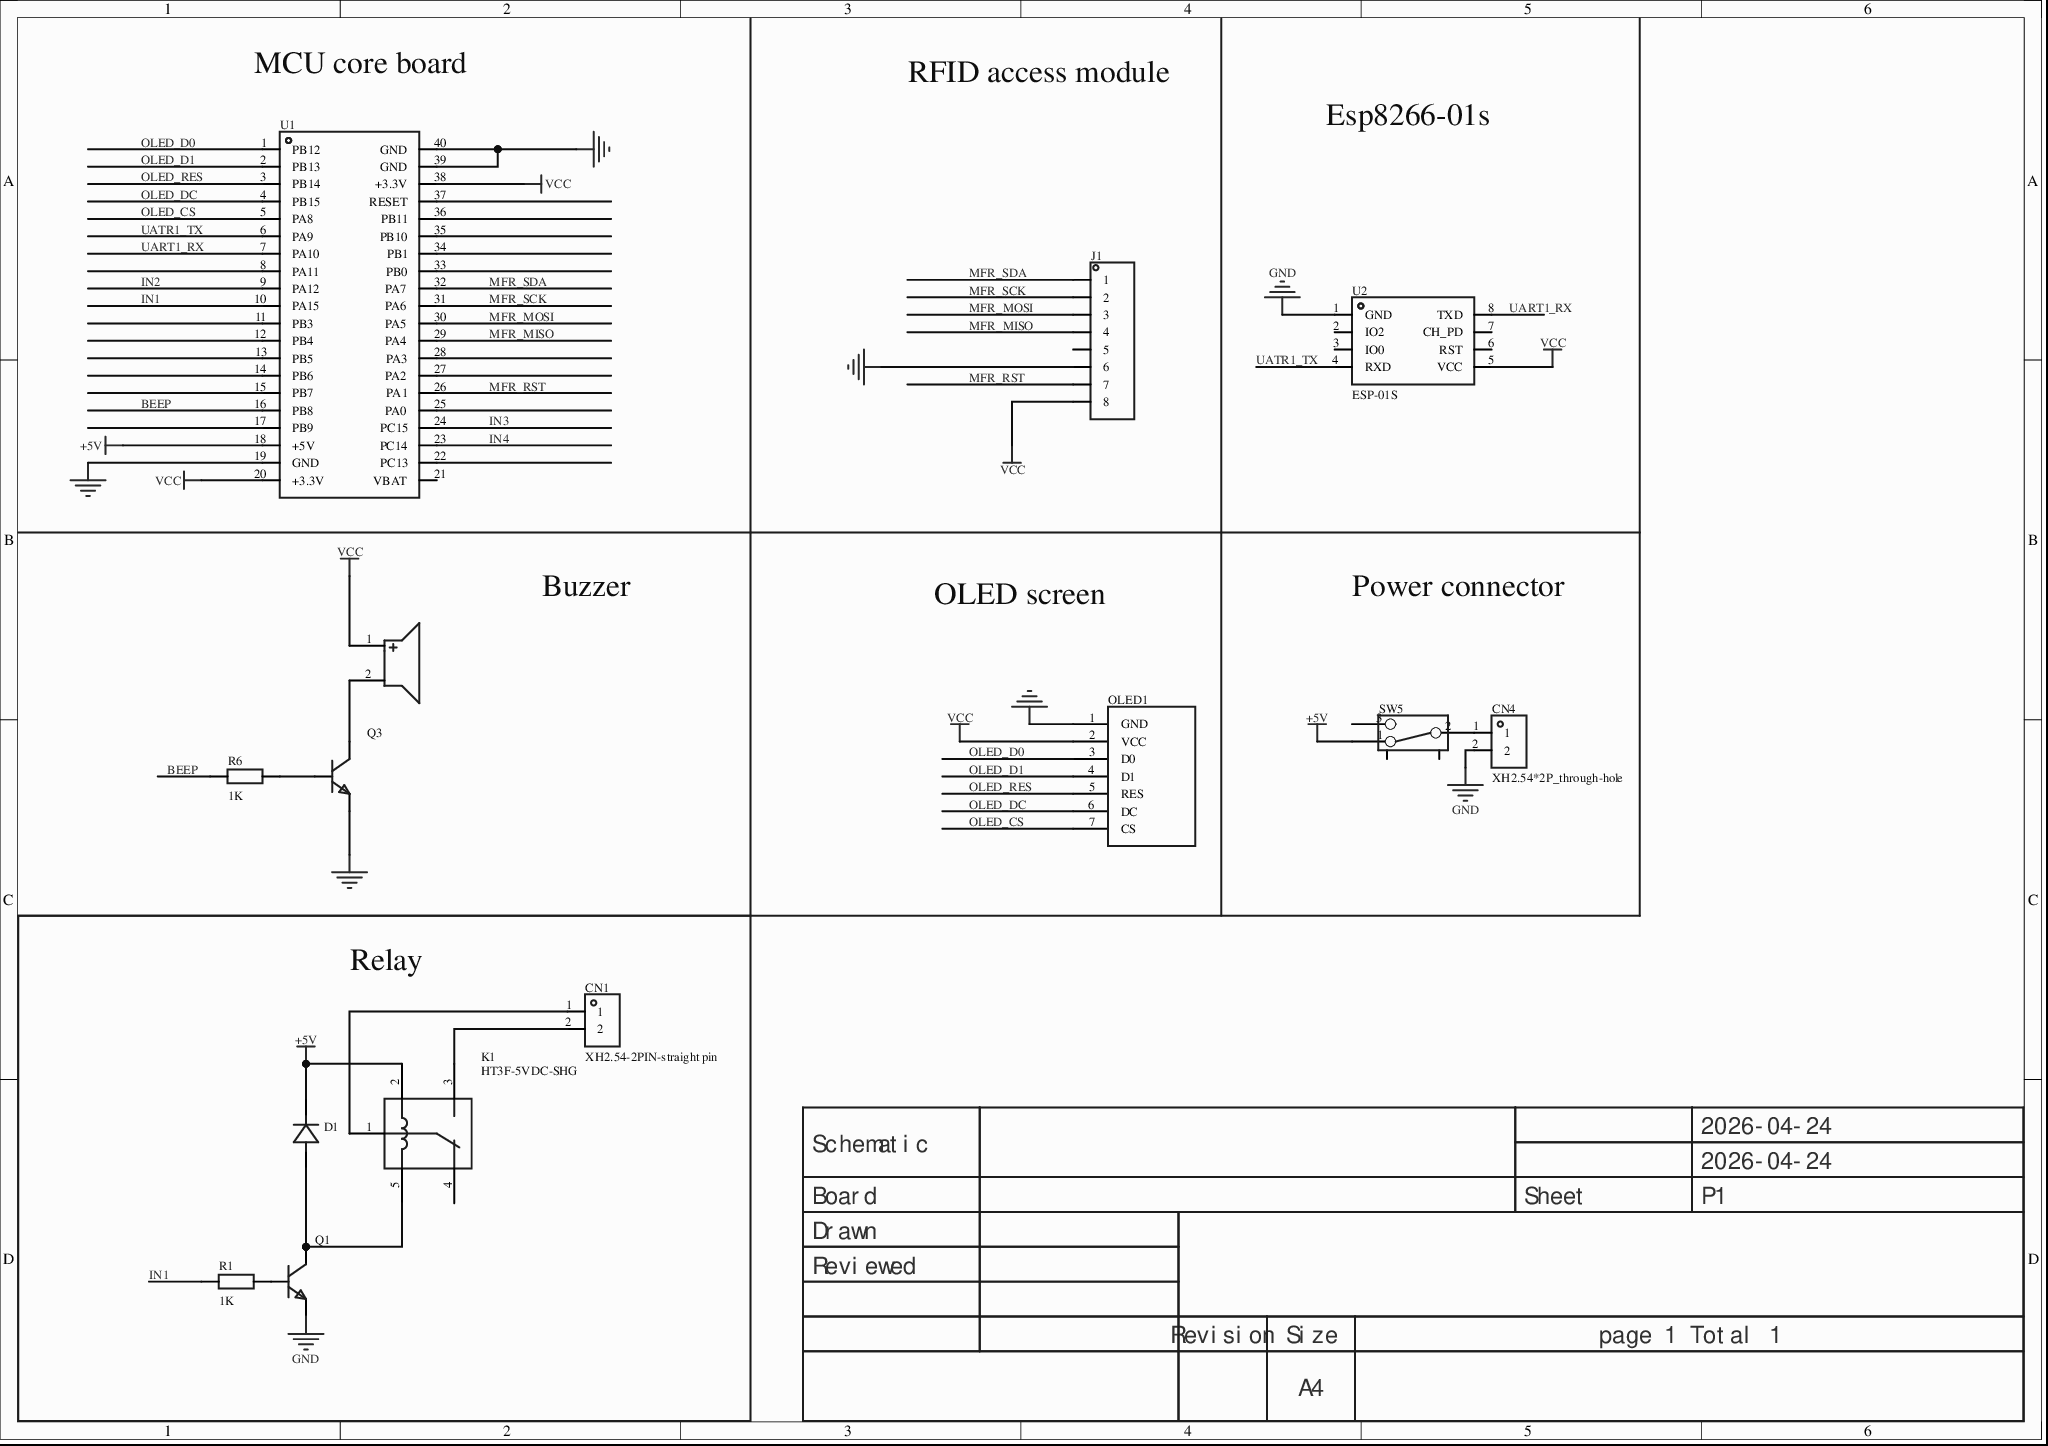
[diagram p0: MISC62443-3.schdoc]
# Altium project MISC62443-2.PrjPcb
1 sheet, 14 parts. Net scope: global (net labels, ports and power ports of the same name join across sheets).
Board file: MISC62443.pcbdoc

## Sheet MISC62443-3.schdoc
size 297 x 209 mm; Version: V1.0; @Project Name: MISC62443; @Page Count: 1; @Update Date: 2026-04-24; @Create Date: 2026-04-24; @Schematic Name: MISC62443; @Page No: 1; @Create Time: 19:02:24; @Update Time: 19:02:29; @Board Name: MISC62443

### Parts
BUZZER1  2.7kHz  [BUZ-TH_BD9.0-P4.00-D0.6-FD]  (value not drawn)
CN1  XH2.54-2PIN-straight pin  [CONN-TH_XH2.54-2P]
CN4  XH2.54*2P_through-hole  [CONN-TH_2P-P2.50-XH2.54-2P]
D1  (no value)  [DO_1N4007]
J1  (no value)  [HDR-TH_8P-P2.54-V-M]
K1  HT3F-5VDC-SHG  [RELAY-TH_HT3F-DCXX-X-X]
OLED1  (no value)  [0.96OLED]
Q1  (no value)  [S8050_SOT-23]
Q3  (no value)  [S8050_TO_92]
R1  1K  [R0603]
R6  1K  [Res_1/8W]
SW5  (no value)  [拨动开关]
U1  LCKFB-DKX-STM32F103C8T6  [CONN-TH_L53.3-W22.9_STM32F103C8T6-CARD]  (value not drawn)
U2  ESP-01S  [WIFIM-TH_ESP-01S]

### Blocks framed on the sheet
Relay: CN1 D1 K1 Q1 R1

### Nets
+5V: D1.1(K) K1.2 SW5.1 U1.18(+5V)
GND: CN4.2 J1.6 OLED1.1(GND) Q1.2 Q3.1(E) U1.19(GND) U1.39(GND) U1.40(GND) U2.1(GND)
VCC: BUZZER1.1 J1.8 OLED1.2(VCC) U1.20(+3.3V) U1.38(+3.3V) U2.5(VCC)
BEEP: R6.1 U1.16(PB8)
IN1: R1.1 U1.10(PA15)
IN2: U1.9(PA12)
IN3: U1.24(PC15)
IN4: U1.23(PC14)
MFR_MISO: J1.4 U1.29(PA4)
MFR_MOSI: J1.3 U1.30(PA5)
MFR_RST: J1.7 U1.26(PA1)
MFR_SCK: J1.2 U1.31(PA6)
MFR_SDA: J1.1 U1.32(PA7)
OLED_CS: OLED1.7(CS) U1.5(PA8)
OLED_D0: OLED1.3(D0) U1.1(PB12)
OLED_D1: OLED1.4(D1) U1.2(PB13)
OLED_DC: OLED1.6(DC) U1.4(PB15)
OLED_RES: OLED1.5(RES) U1.3(PB14)
UART1_RX: U1.7(PA10) U2.8(TXD)
UATR1_TX: U1.6(PA9) U2.4(RXD)
NetBUZZER1_2: BUZZER1.2 Q3.3(C)
NetCN1_1: CN1.1 K1.1
NetCN1_2: CN1.2 K1.3
NetCN4_1: CN4.1 SW5.2
NetD1_2: D1.2(A) K1.5 Q1.3
NetQ1_1: Q1.1 R1.2
NetQ3_2: Q3.2(B) R6.2

Not connected (* = marked no-connect by the designer): J1 5; K1 4*; SW5 3 4 5; U1 8(PA11) 11(PB3) 12(PB4) 13(PB5) 14(PB6) 15(PB7) 17(PB9) 21(VBAT) 22(PC13) 25(PA0) 27(PA2) 28(PA3) 33(PB0) 34(PB1) 35(PB10) 36(PB11) 37(RESET); U2 2(IO2)* 3(IO0)* 6(RST)* 7(CH_PD)*

### Notes on the sheet
- MCU core board
- RFID access module
- Esp8266-01s
- Buzzer
- OLED screen
- Power connector
- 2026-04-24
- Schematic
- Board
- Sheet
- P1
- Drawn
- Reviewed
- Revision
- Size
- A4
- page 1 Total 1

### Library data of the parts
BUZZER1 = QMB-09B-03: Drive: passive (external drive); type: electromagnetic; frequency: 2.7kHz; SPL: 85dB;; Manufacturer: 华能; AddInBom: yes; ModelId: 949096c5110a440bbcfd89e7e6948986; ModelName: BUZ-TH_D9.0-H5.5-P4.0; ModelTransform: 354.33,354.33,0,90,0,0,0,0,-177.165; Voltage - Supply: 2V~5V; Symbol: QMB-09B-03; Device: QMB-09B-03; LCSC Part Name: 无源蜂鸣器QMB-09B-03; SupplierPart: C96256; ManufacturerPart: QMB-09B-03; Supplier Footprint: 插件,D=9mm; JLCPCB Part Class: Extended library; Datasheet: https://atta.szlcsc.com/upload/public/pdf/source/20210401/C96256_958B17753B5AD7CBFBCFFC7C095B4484.pdf; Supplier: LCSC; ConvertToPcb: yes; FootprintName: BUZ-TH_BD9.0-P4.00-D0.6-FD; Driver Circuitry: Passive (external drive); Technology: Electromagnetic; Value: 2.7kHz; Sound Pressure Level(SPL): 85dB; Diameter(φD): 9mm; Height: 5.7mm
CN1 = XH2.54-2PIN-直针: AddInBom: yes; ModelId: c3cc11bd8b8748c1ae6bc231aac3a1ff0819f05c4eef4c71ace90d822a990e87; ModelTransform: 296.889,230.315,0,0,0,0,0,26.653,-137.795; Symbol: XH2.54-2PIN-straight pin; Device: XH2.54-2PIN-straight pin; LCSC Part Name: XH2.54-2PIN-直针; SupplierPart: C9900011425; ManufacturerPart: XH2.54-2PIN-直针; Supplier Footprint: XH2.54-2PIN; JLCPCB Part Class: Extended Part; Supplier: LCSC; ConvertToPcb: yes; FootprintName: CONN-TH_XH2.54-2P; ModelName: CONN-TH_XH2.54-2P
CN4 = XH2.54*2P_直插: 3D Model: 325c595e30db4df8abe76612dd40b0fa0819f05c4eef4c71ace90d822a990e87; 3D Model Transform: 295.275,228.346,0,180,0,0,-0.002,-20.079,-137.795; AddInBom: yes; Symbol: XH2.54*2P_through-hole; Device: XH2.54*2P_through-hole; LCSC Part Name: XH2.54*2P_直插; Supplier Part: C9900008615; Manufacturer Part: XH2.54*2P_直插; Supplier Footprint: XH2.54_2P; JLCPCB Part Class: Extended Part; Supplier: LCSC; FootprintName: CONN-TH_2P-P2.50-XH2.54-2P; ConvertToPcb: yes; ModelName: CONN-TH_2P-P2.50-XH2.54-2P
D1 = D_1N4007A: AddInBom: yes; ModelId: 6de1e9b71a0d4751b4e9df530304c1a3; ModelName: DO-41_D2.4-L4.7-P8.70; ModelTransform: 373.9,94.4,232.29,0,0,0,0,0,-140; Symbol: D_1N4007; Device: D_1N4007A; Supplier Footprint: DO-41; ConvertToPcb: yes; FootprintName: DO_1N4007
J1 = HDR-M_2.54_1x8P: Symbol: Header-Male-2.54_1x8; ConvertToPcb: yes; ModelId: f5b96e27511e49e38545e53df2320202; ModelTransform: 807.87244,98.425,0,0,0,0,0,0,-118.11; Device: HDR-M_2.54_1x8P; AddInBom: yes; SupplierPart: C124381; Supplier Footprint: 插件; FootprintName: HDR-TH_8P-P2.54-V-M; ModelName: HDR-TH_8P-P2.54-V-M
K1 = HT3F-5VDC-SHG: Coil voltage: 5V; contact form: changeover: 1C (SPDT); contact rating (resistive load): 10A@120VAC; 10A@277VAC; 10A@30VDC; max switching voltage: -; max switching current: -; Manufacturer: HTV(博粤); AddInBom: yes; ModelId: c9d4d8384bf9459d8ed312453b321f1c0819f05c4eef4c71ace90d822a990e87; ModelTransform: 748.03,610.235,0,0,0,0,35.394,0,-137.795; Coil Rated Power: 360mW; Coil Resistance: 70Ω; Contact Resistance: 100mΩ; Operate Time: 10ms; Release Time: 5ms; Symbol: HT3F-5VDC-SHG; Device: HT3F-5VDC-SHG; LCSC Part Name: 继电器; SupplierPart: C129113; ManufacturerPart: HT3F-5VDC-SHG; Supplier Footprint: 插件,19x15.5mm; JLCPCB Part Class: Extended Part; Datasheet: https://item.szlcsc.com/datasheet/HT3F-5VDC-SHG/140399.html; Supplier: LCSC; ConvertToPcb: yes; FootprintName: RELAY-TH_HT3F-DCXX-X-X; ModelName: RELAY-TH_HT3F-DCXX-X-X; Coil Voltage: 5V; Contact Form: Changeover: 1C (SPDT); Number of Pins: -; Contact Rating: 10A@120VAC; 10A@277VAC; 10A@30VDC; Switching Voltage(Max): -; Contact Material: -; Switching Current(Max): -; Coil Type: -; Operating Temperature: -40℃~+70℃
OLED1 = 0.96OLED: AddInBom: yes; _: 3; Device: 0.96OLED; ConvertToPcb: yes; SymbolName: 0.96OLED; FootprintName: 0.96OLED
Q1 = S8050_SOT_NPN: Symbol: NPN; ConvertToPcb: yes; ModelId: c62791f0466c4ae2a892c056b845b0ca0819f05c4eef4c71ace90d822a990e87; ModelName: SOT-23-3P_L2.9-W1.3-H1.0-LS2.4-P0.95; ModelTransform: 98.6,114.12,41.29,180,0,0,0,0,-3; Device: S8050_SOT_NPN; AddInBom: yes; Supplier Footprint: SOT-23; FootprintName: S8050_SOT-23
Q3 = S8050_TO_NPN: ConvertToPcb: yes; ModelId: aafe8e06f2154e7c93506efd0d6632dd; ModelName: TO-92-3_L4.9-W3.7-P1.27-L; ModelTransform: 180.78,141.44,417.3,0,0,0,0,0,-200; Device: S8050_TO_NPN; AddInBom: yes; Supplier Footprint: TO-92; SymbolName: S8050_TO_NPN; FootprintName: S8050_TO_92
R1 = Res_0603: Symbol: Resistor; ConvertToPcb: yes; ModelId: fc143cca1e79419f9cd78b61e9279f080819f05c4eef4c71ace90d822a990e87; ModelTransform: 31.8897,63.7794,0,90,0,0,0,0,0; Device: Res_0603; Value: 1K; AddInBom: yes; Supplier Footprint: 0603; FootprintName: R0603; ModelName: R0603
R6 = Res_AXIAL-1/8W: ConvertToPcb: yes; SymbolName: Resistor; ModelId: b2b5ae7ae4c642178fe0039925c86a3f; ModelName: RES-TH_BD1.8-L3.2-P7.20-D0.4; ModelTransform: 282.86,66.88,253.09,0,0,0,0,0,-191; Value: 1K; Device: Res_AXIAL-1/8W; AddInBom: yes; Supplier Footprint: 轴向引线; FootprintName: Res_1/8W
SW5 = 拨动开关_正: Symbol: Toggle switch; Device: Toggle switch_positive; 3D Model: 4321fe59a4074cbfb4989553f297c68f0819f05c4eef4c71ace90d822a990e87; 3D Model Transform: 370.09,208.7,472.35,0,0,0,0,0,-110; ConvertToPcb: yes; ModelName: SW-TH_SS-12D02-VG4; Supplier Footprint: 插件; FootprintName: Toggle switch; AddInBom: yes
U1 = LCKFB-DKX-STM32F103C8T6: Manufacturer: 立创开发板; AddInBom: yes; Symbol: LCKFB-DKX-STM32F103C8T6; Device: LCKFB-DKX-STM32F103C8T6; LCSC Part Name: 立创·地阔星-STM32F103C8T6开发板; SupplierPart: C22396880; ManufacturerPart: LCKFB-DKX-STM32F103C8T6; Supplier Footprint: -; JLCPCB Part Class: Extended library; Datasheet: https://atta.szlcsc.com/upload/public/pdf/source/20240801/7EEF69F7480DF7C6DA98696664D658D4.pdf; Supplier: LCSC; ConvertToPcb: yes; FootprintName: CONN-TH_L53.3-W22.9_STM32F103C8T6-CARD
U2 = ESP-01S_C111009: 3D Model: eb7175da78ae48b3b1568cfe3027405f0819f05c4eef4c71ace90d822a990e87; 3D Model Transform: 582.676,976.37608,0,0,0,0,0,388.346,-118.11; AddInBom: yes; Symbol: ESP-01S; Device: ESP-01S_C111009; LCSC Part Name: ESP-01S; Supplier Part: C111009; Manufacturer Part: ESP-01S; Supplier Footprint: -; JLCPCB Part Class: Extended Part; Supplier: LCSC; ConvertToPcb: yes; FootprintName: WIFIM-TH_ESP-01S; ModelName: WIFIM-TH_ESP-01S